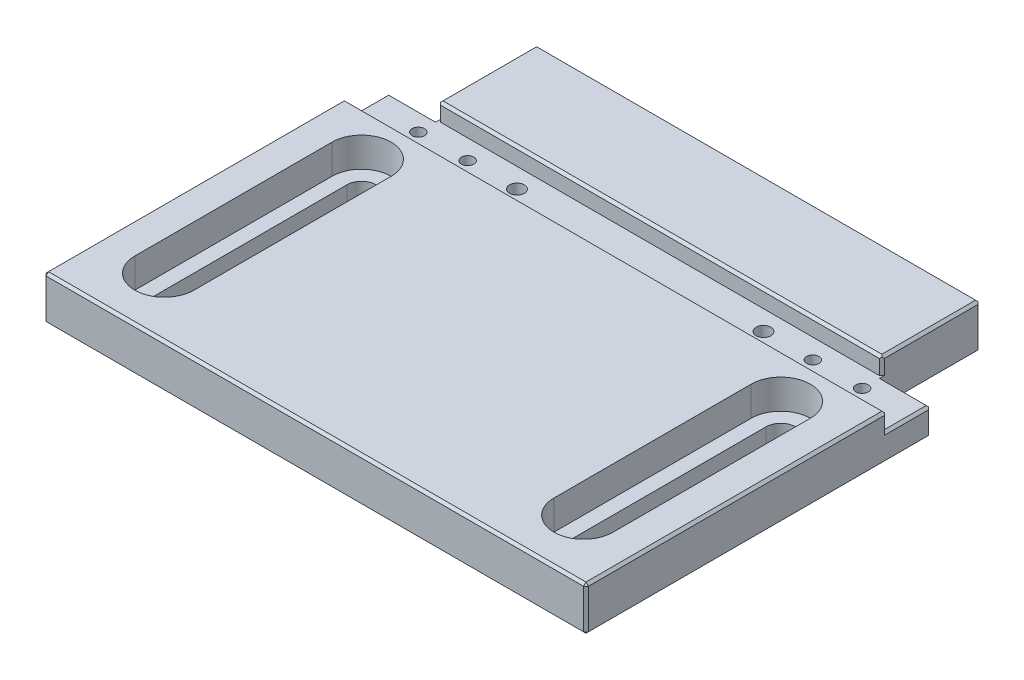
from build123d import *

# Parameters (mm, degrees)
SKETCH1_W             = 110
SKETCH1_H             = 90
BOSS_EXTRUDE1_DEPTH   = 9
SKETCH2_W             = 110
SKETCH2_H             = 8
BOSS_EXTRUDE2_DEPTH   = 1.5
SKETCH5_W             = 20
SKETCH5_H             = 20
BOSS_EXTRUDE3_DEPTH   = 9
CUT_EXTRUDE1_DEPTH    = 156.823618235
CUT_EXTRUDE2_DEPTH    = 6
SKETCH6_W             = 10
SKETCH6_H             = 40
CUT_EXTRUDE3_DEPTH    = 156.823618235
SKETCH8_W             = 110
SKETCH8_H             = 9
CUT_EXTRUDE5_DEPTH    = 5
M3_TAPPED_HOLE1_D     = 2.5
MOVE_FACE1_BY         = 20
MOVE_FACE1_2_BY       = 20
F_3_0MM_DOWEL_HOLE1_D = 3
CHAMFER1_SIZE         = 0.5
CHAMFER3_SIZE         = 0.5
CHAMFER4_SIZE         = 0.5


with BuildPart() as part:
    # Sketch1 → Boss-Extrude1 (new body)
    with BuildSketch(Plane(origin=(0, 0, 0), x_dir=(1, 0, 0), z_dir=(0, 1, 0))):
        with Locations((55, 45)):
            Rectangle(SKETCH1_W, SKETCH1_H)
    extrude(amount=BOSS_EXTRUDE1_DEPTH)

    # Sketch2 → Boss-Extrude2 (add)
    with BuildSketch(Plane(origin=(0, 9, 0), x_dir=(1, 0, 0), z_dir=(0, 1, 0))):
        with Locations((55, 66)):
            Rectangle(SKETCH2_W, SKETCH2_H)
    extrude(amount=BOSS_EXTRUDE2_DEPTH)

    # Sketch5 → Boss-Extrude3 (add)
    with BuildSketch(Plane.XZ):
        with Locations((10, -100)):
            Rectangle(SKETCH5_W, SKETCH5_H)
        with Locations((100, -100)):
            Rectangle(SKETCH5_W, SKETCH5_H)
    extrude(amount=-BOSS_EXTRUDE3_DEPTH)

    # Sketch3 → Cut-Extrude1 (cut, through all)
    with BuildSketch(Plane(origin=(0, 9, 0), x_dir=(1, 0, 0), z_dir=(0, 1, 0))):
        with BuildLine():
            Line((15.5, 52), (15.5, 12))
            ThreePointArc((15.5, 12), (12.5, 9), (9.5, 12))
            Line((9.5, 12), (9.5, 52))
            ThreePointArc((9.5, 52), (12.5, 55), (15.5, 52))
        make_face()
        with BuildLine():
            Line((94.5, 52), (94.5, 12))
            ThreePointArc((94.5, 12), (97.5, 9), (100.5, 12))
            Line((100.5, 12), (100.5, 52))
            ThreePointArc((100.5, 52), (97.5, 55), (94.5, 52))
        make_face()
    extrude(amount=-CUT_EXTRUDE1_DEPTH, mode=Mode.SUBTRACT)

    # Sketch4 → Cut-Extrude2 (cut)
    with BuildSketch(Plane(origin=(0, 9, 0), x_dir=(1, 0, 0), z_dir=(0, 1, 0))):
        with BuildLine():
            Line((6.5, 52), (6.5, 12))
            ThreePointArc((6.5, 12), (12.5, 6), (18.5, 12))
            Line((18.5, 12), (18.5, 52))
            ThreePointArc((18.5, 52), (12.5, 58), (6.5, 52))
        make_face()
        with BuildLine():
            Line((103.5, 12), (103.5, 52))
            ThreePointArc((103.5, 52), (97.5, 58), (91.5, 52))
            Line((91.5, 52), (91.5, 12))
            ThreePointArc((91.5, 12), (97.5, 6), (103.5, 12))
        make_face()
    extrude(amount=-CUT_EXTRUDE2_DEPTH, mode=Mode.SUBTRACT)

    # Sketch6 → Cut-Extrude3 (cut, through all)
    with BuildSketch(Plane(origin=(0, 9, 0), x_dir=(1, 0, 0), z_dir=(0, 1, 0))):
        with Locations((5, 90)):
            Rectangle(SKETCH6_W, SKETCH6_H)
        with Locations((105, 90)):
            Rectangle(SKETCH6_W, SKETCH6_H)
    extrude(amount=-CUT_EXTRUDE3_DEPTH, mode=Mode.SUBTRACT)

    # Sketch8 → Cut-Extrude5 (cut)
    with BuildSketch(Plane(origin=(0, 10.5, 0), x_dir=(1, 0, 0), z_dir=(0, 1, 0))):
        with Locations((55, 65.5)):
            Rectangle(SKETCH8_W, SKETCH8_H)
    extrude(amount=-CUT_EXTRUDE5_DEPTH, mode=Mode.SUBTRACT)

    # M3 Tapped Hole1 (through all)
    with Locations(Plane(origin=(0, 5.5, 0), x_dir=(1, 0, 0), z_dir=(0, 1, 0))):
        with Locations((10, 66), (100, 66), (20, 66), (90, 66)):
            Hole(M3_TAPPED_HOLE1_D / 2)

    # Move Face1: a face moved inward by 20.0
    extrude(part.faces().sort_by_distance((95, 4.5, -110))[0], amount=MOVE_FACE1_BY, dir=(0, 0, 1), mode=Mode.SUBTRACT)

    # Move Face1 2: a face moved inward by 20.0
    extrude(part.faces().sort_by_distance((15, 4.5, -110))[0], amount=MOVE_FACE1_2_BY, dir=(0, 0, 1), mode=Mode.SUBTRACT)

    # Ø3.0mm dowel hole1 (through all)
    with Locations(Plane(origin=(0, 5.5, 0), x_dir=(1, 0, 0), z_dir=(0, 1, 0))):
        with Locations((30, 66), (80, 66)):
            Hole(F_3_0MM_DOWEL_HOLE1_D / 2)

    # Chamfer1
    chamfer1_edges = [part.edges().sort_by_distance(p)[0] for p in [
        (0, 0, -35),
        (110, 9, -30.5),
        (10, 4.5, -90),
        (100, 4.5, -90),
        (110, 2.75, -70),
        (0, 2.75, -70),
        (0, 9, -30.5),
        (110, 7.25, -61),
        (0, 7.25, -61),
        (0, 5.5, -65.5),
        (110, 5.5, -65.5),
        (55, 9, -90),
        (55, 0, -90),
        (110, 0, -35),
        (55, 0, 0),
        (110, 4.5, 0),
        (0, 4.5, 0),
        (55, 9, 0),
    ]]
    chamfer(chamfer1_edges, length=CHAMFER1_SIZE)

    # Chamfer3
    chamfer3_edges = [part.edges().sort_by_distance(p)[0] for p in [
        (55, 9, -70),
        (10, 0, -79.75),
        (10, 9, -79.75),
        (104.75, 0, -70),
        (5.25, 5.5, -70),
        (100, 0, -79.75),
        (5.25, 0, -70),
        (100, 9, -79.75),
        (104.75, 5.5, -70),
        (55, 9, -61),
    ]]
    chamfer(chamfer3_edges, length=CHAMFER3_SIZE)

    # Chamfer4
    chamfer4_edges = [part.edges().sort_by_distance(p)[0] for p in [
        (10, 7, -70),
        (100, 7, -70),
    ]]
    chamfer(chamfer4_edges, length=CHAMFER4_SIZE)


solid = part.part
